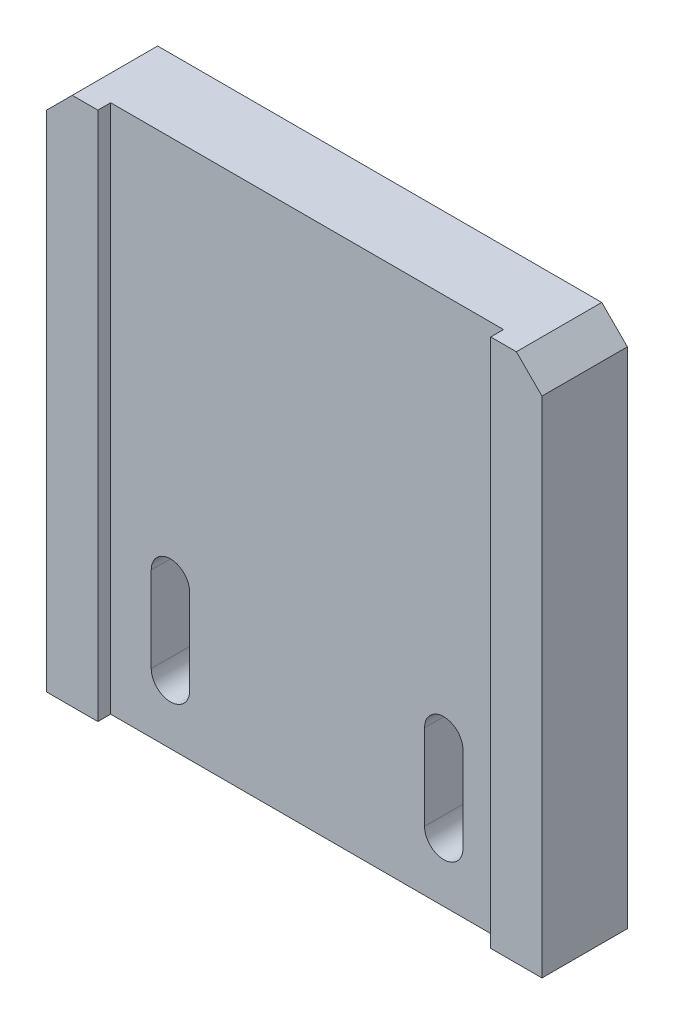
from build123d import *

# Parameters (mm, degrees)
SKETCH_1_W          = 58
SKETCH_1_H          = 62
EXTRUDE_1_DEPTH     = 10
SKETCH_2_W          = 46
SKETCH_2_H          = 62
CUT_EXTRUDE_1_DEPTH = 1.5
CHAMFER_1_SIZE      = 3
CUT_EXTRUDE_2_REACH = 45.293


with BuildPart() as part:
    # 草图1 → 凸台-拉伸1 (new body)
    with BuildSketch(Plane.XY):
        Rectangle(SKETCH_1_W, SKETCH_1_H)
    extrude(amount=EXTRUDE_1_DEPTH)

    # 草图2 → 切除-拉伸1 (cut)
    with BuildSketch(Plane.XY.offset(10)):
        Rectangle(SKETCH_2_W, SKETCH_2_H)
    extrude(amount=-CUT_EXTRUDE_1_DEPTH, mode=Mode.SUBTRACT)

    # 倒角1
    chamfer_1_edges = [part.edges().sort_by_distance(p)[0] for p in [
        (-29, 31, 5),
        (29, 31, 5),
    ]]
    chamfer(chamfer_1_edges, length=CHAMFER_1_SIZE)

    # 草图3 → 切除-拉伸2 (cut, up to next)
    with BuildSketch(Plane.XY.offset(8.5), mode=Mode.PRIVATE) as cut_extrude_2_sk1:
        with BuildLine():
            Line((-18.25, -24), (-18.25, -14))
            ThreePointArc((-18.25, -14), (-16, -11.75), (-13.75, -14))
            Line((-13.75, -14), (-13.75, -24))
            ThreePointArc((-13.75, -24), (-16, -26.25), (-18.25, -24))
        make_face()
    cut_extrude_2_tool1 = extrude(cut_extrude_2_sk1.sketch, amount=-CUT_EXTRUDE_2_REACH, mode=Mode.PRIVATE) & part.part
    cut_extrude_2 = cut_extrude_2_tool1.solids().sort_by_distance((-16, -19, 8.5))[0]
    add(cut_extrude_2, mode=Mode.SUBTRACT)

    # 镜向1: 切除-拉伸2 across plane
    add(cut_extrude_2.mirror(Plane(origin=(0, 0, 0), x_dir=(0, 0, 1), z_dir=(1, 0, 0))), mode=Mode.SUBTRACT)


solid = part.part
